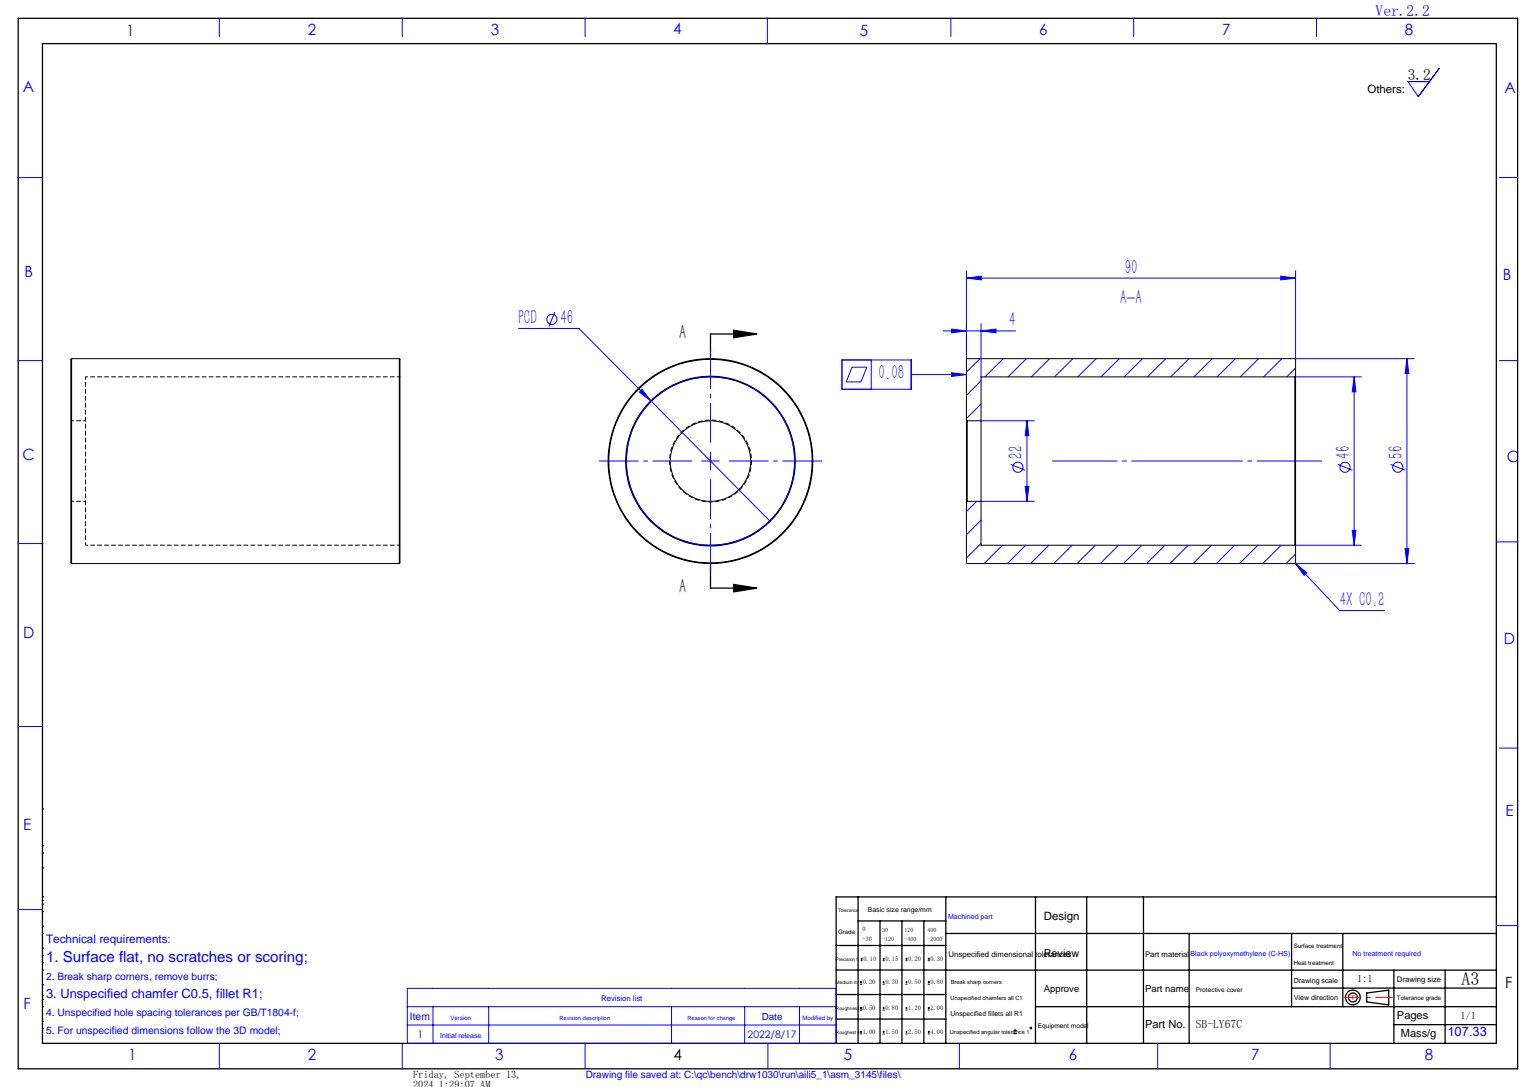
from build123d import *

# Parameters (mm, degrees)
SKETCH_3_R      = 28
SKETCH_3_R_2    = 23
EXTRUDE_1_DEPTH = 90
SKETCH_4_R      = 23.5
SKETCH_4_R_2    = 11
EXTRUDE_2_DEPTH = 4
CHAMFER_1_SIZE  = 0.2


with BuildPart() as part:
    # 草图3 → 凸台-拉伸1 (new body)
    with BuildSketch(Plane(origin=(0, 0, 0), x_dir=(1, 0, 0), z_dir=(0, 1, 0))):
        with Locations(Location((0, 0, 0), (0, 0, 90))):
            Circle(SKETCH_3_R)
        with Locations(Location((0, 0, 0), (0, 0, 90))):
            Circle(SKETCH_3_R_2, mode=Mode.SUBTRACT)
    extrude(amount=EXTRUDE_1_DEPTH)

    # 草图4 → 凸台-拉伸2 (add)
    with BuildSketch(Plane.XZ.offset(-90)):
        Circle(SKETCH_4_R)
        with Locations(Location((0, 0, 0), (0, 0, 270))):
            Circle(SKETCH_4_R_2, mode=Mode.SUBTRACT)
    extrude(amount=EXTRUDE_2_DEPTH)

    # 倒角1
    chamfer_1_edges = [part.edges().sort_by_distance(p)[0] for p in [
        (0, 90, 11),
        (0, 0, 28),
        (0, 90, 28),
        (0, 0, 23),
    ]]
    chamfer(chamfer_1_edges, length=CHAMFER_1_SIZE)


solid = part.part
